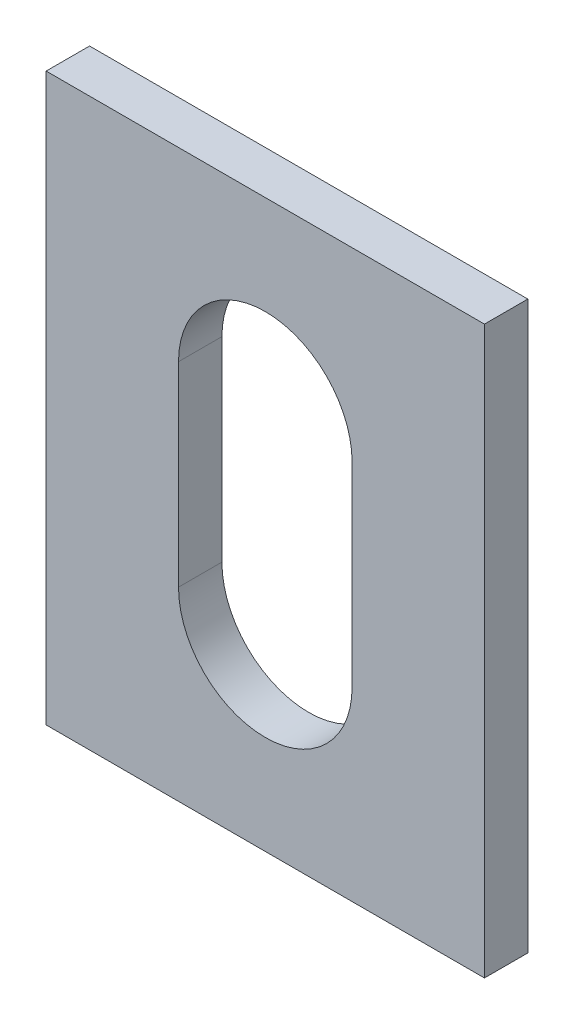
from build123d import *

# Parameters (mm, degrees)
SKETCH_1_W          = 202
SKETCH_1_H          = 261
EXTRUDE_1_DEPTH     = 20
CUT_EXTRUDE_1_DEPTH = 378.710206375


with BuildPart() as part:
    # 草图1 → 凸台-拉伸1 (new body)
    with BuildSketch(Plane.XY):
        with Locations((-176, -125.5)):
            Rectangle(SKETCH_1_W, SKETCH_1_H)
    extrude(amount=EXTRUDE_1_DEPTH)

    # 草图2 → 切除-拉伸1 (cut, through all)
    with BuildSketch(Plane.XY.offset(20)):
        with BuildLine():
            Line((-216, -170.5), (-216, -80.5))
            ThreePointArc((-216, -80.5), (-176, -40.5), (-136, -80.5))
            Line((-136, -80.5), (-136, -170.5))
            ThreePointArc((-136, -170.5), (-176, -210.5), (-216, -170.5))
        make_face()
    extrude(amount=-CUT_EXTRUDE_1_DEPTH, mode=Mode.SUBTRACT)


solid = part.part
